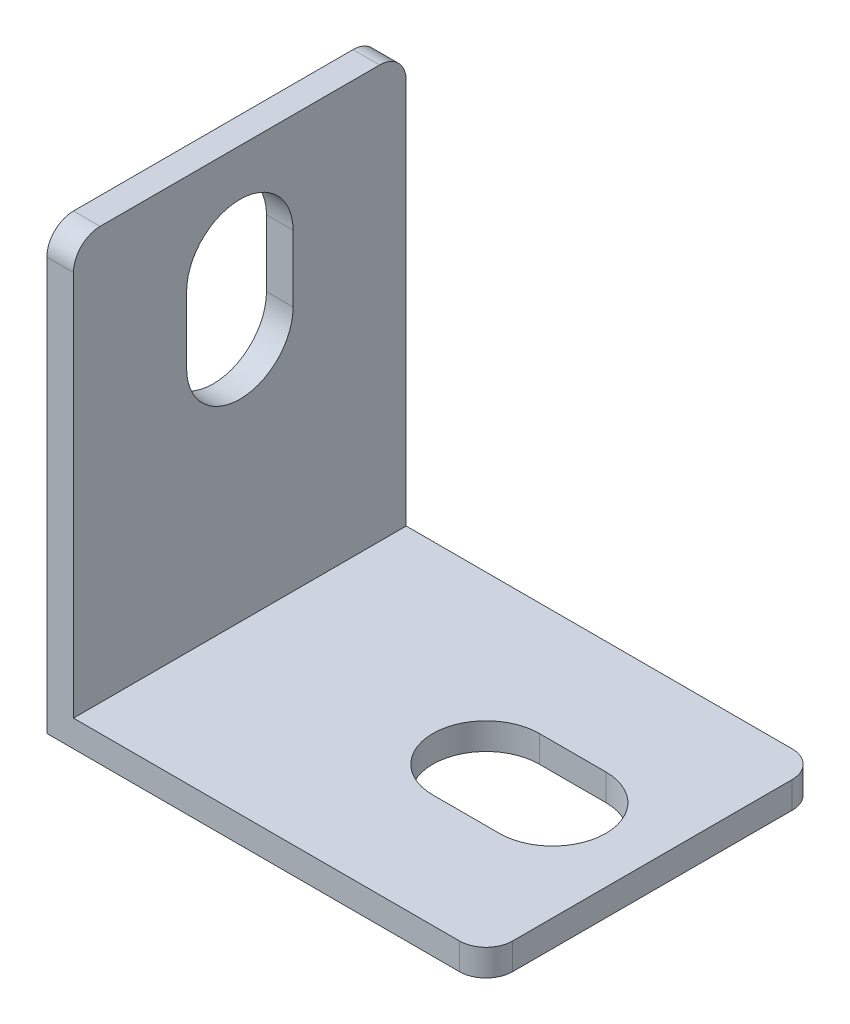
from build123d import *

# Parameters (mm, degrees)
EXTRUDE_1_DEPTH     = 25
FILLET_1_R          = 2
CUT_EXTRUDE_1_DEPTH = 52.720402164
CUT_EXTRUDE_2_DEPTH = 52.720402164


with BuildPart() as part:
    # 草图1 → 凸台-拉伸1 (new body)
    with BuildSketch(Plane.XY):
        Polygon((0, 0), (33, 0), (33, 2), (2, 2), (2, 33), (0, 33), align=None)
    extrude(amount=EXTRUDE_1_DEPTH)

    # 圆角1
    fillet_1_edges = [part.edges().sort_by_distance(p)[0] for p in [
        (33, 1, 25),
        (1, 33, 25),
        (1, 33, 0),
        (33, 1, 0),
    ]]
    fillet(fillet_1_edges, radius=FILLET_1_R)

    # 草图2 → 切除-拉伸1 (cut, through all)
    with BuildSketch(Plane(origin=(0, 2, 0), x_dir=(1, 0, 0), z_dir=(0, 1, 0))):
        with BuildLine():
            Line((20.5, -8.5), (25.5, -8.5))
            ThreePointArc((25.5, -8.5), (29.5, -12.5), (25.5, -16.5))
            Line((25.5, -16.5), (20.5, -16.5))
            ThreePointArc((20.5, -16.5), (16.5, -12.5), (20.5, -8.5))
        make_face()
    extrude(amount=-CUT_EXTRUDE_1_DEPTH, mode=Mode.SUBTRACT)

    # 草图4 → 切除-拉伸2 (cut, through all)
    with BuildSketch(Plane(origin=(2, 0, 0), x_dir=(0, 0, -1), z_dir=(1, 0, 0))):
        with BuildLine():
            Line((-8.5, 25.5), (-8.5, 20.5))
            ThreePointArc((-8.5, 20.5), (-12.5, 16.5), (-16.5, 20.5))
            Line((-16.5, 20.5), (-16.5, 25.5))
            ThreePointArc((-16.5, 25.5), (-12.5, 29.5), (-8.5, 25.5))
        make_face()
    extrude(amount=-CUT_EXTRUDE_2_DEPTH, mode=Mode.SUBTRACT)


solid = part.part
